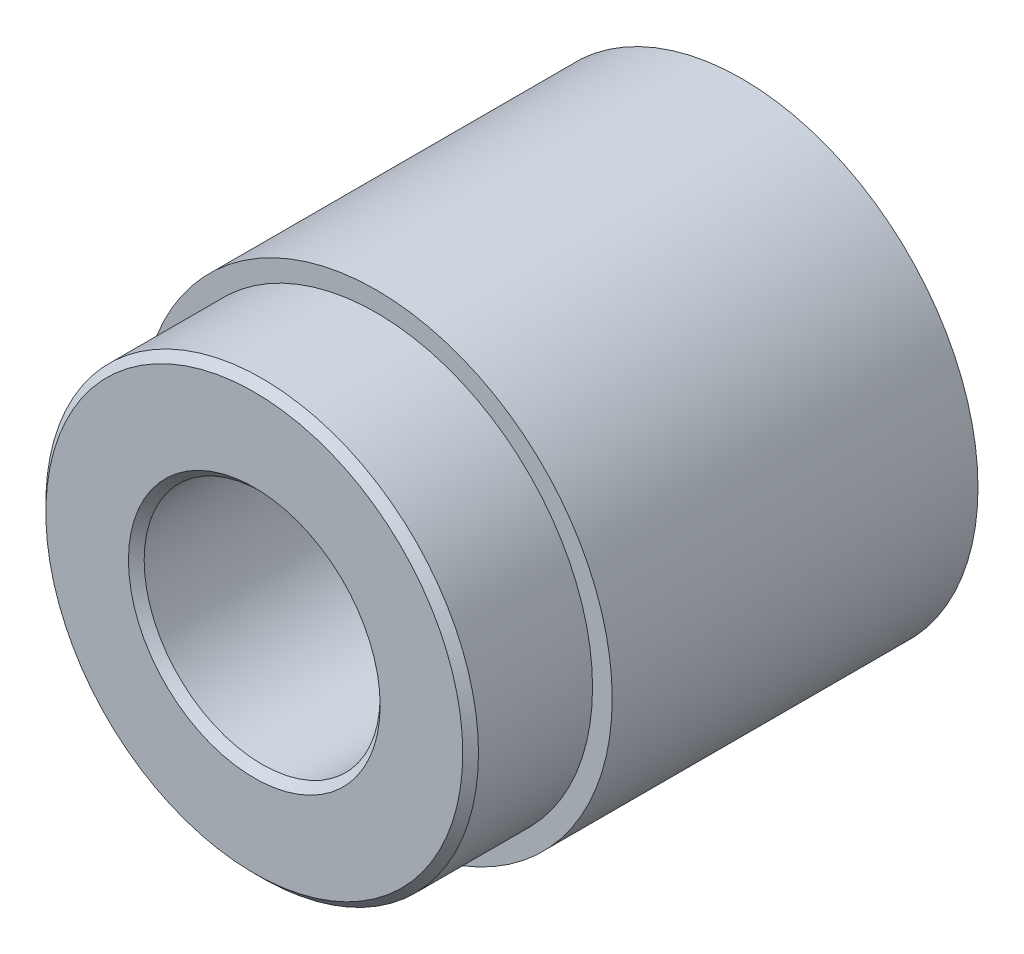
SolidWorks part; units mm, degrees
ref_plane "Front Plane" through (0, 0, 0) normal (0, 0, 1) x (1, 0, 0)
ref_plane "Top Plane" through (0, 0, 0) normal (0, 1, 0) x (1, 0, 0)
ref_plane "Right Plane" through (0, 0, 0) normal (1, 0, 0) x (0, 0, -1)
sketch "Sketch1" plane through (0, 0, 0) normal (0, 0, 1) x (1, 0, 0)
  circle A0 centre (0, 0) radius 30
  circle A1 centre (0, 0) radius 60
  dimension "D1" = 60
  dimension "D2" = 120
extrude "Boss-Extrude1" add sketch "Sketch1" along normal blind 124
sketch "Sketch2" plane through (0, 0, 124) normal (0, 0, 1) x (1, 0, 0)
  circle A0 centre (0, 0) radius 55
  circle A1 centre (0, 0) radius 60 construction
  circle A2 centre (0, 0) radius 60
  dimension "D1" = 110
extrude "Cut-Extrude1" cut sketch "Sketch2" against normal blind 31
chamfer "Chamfer1" distance 2 angle 45 3 edges at (30, 0, 0) (55, 0, 124) (30, 0, 124)
